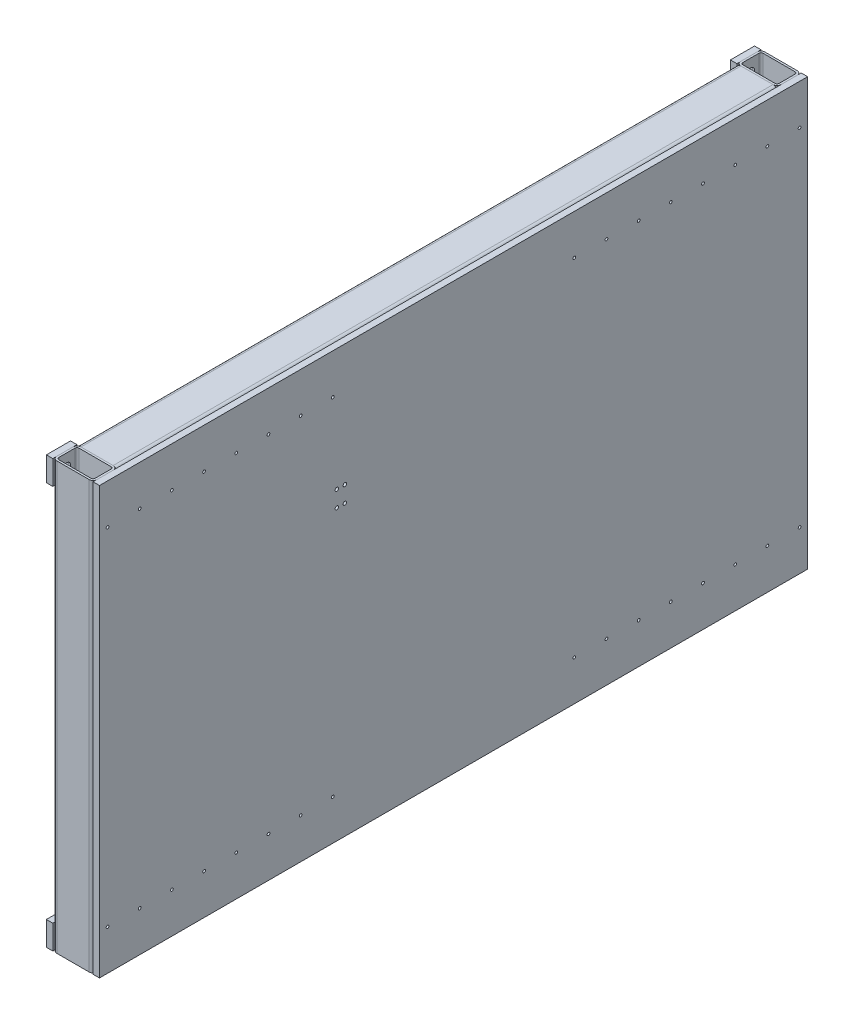
from build123d import *

# Parameters (mm, degrees)
F_100_X_60_X_5_0_1_DEPTH      = 1030
F_100_X_60_X_5_0_1_DEPTH_BACK = 30
F_100_X_60_X_5_0_1_2_DEPTH    = 1060
F_100_X_60_X_5_0_1_3_DEPTH    = 1702
F_100_X_60_X_5_0_1_4_DEPTH    = 1702
F_100_X_60_X_5_0_1_5_DEPTH    = 1702
F_100_X_60_X_5_0_1_6_DEPTH    = 1702
SKETCH_4_W                    = 1760
SKETCH_4_H                    = 1060
EXTRUDE_1_DEPTH               = 16
SKETCH_5_W                    = 60
SKETCH_5_H                    = 60
EXTRUDE_2_DEPTH               = 16
EXTRUDE_2_2_DEPTH             = 16
PATTERN_LINEAR_1_COUNT        = 8
PATTERN_LINEAR_1_PITCH        = 80
HOLE_WIZARD_M10_1_AT_2_COUNT  = 2
HOLE_WIZARD_M10_1_AT_2_PITCH  = 40
HOLE_WIZARD_M10_1_AT_3_COUNT  = 2
HOLE_WIZARD_M10_1_AT_3_PITCH  = 20
HOLE_WIZARD_M10_1_AT_4_COUNT  = 2
HOLE_WIZARD_M10_1_AT_4_PITCH  = 44.72135955


with BuildPart() as part:
    # Sketch1 → 矩型管 100 X 60 X 5.0(1) (new, two sides: drawn at the far end of the back side and taken through both)
    with BuildSketch(Plane(origin=(0, 500, 850), x_dir=(0, 0, -1), z_dir=(0, -1, 0)).offset(-F_100_X_60_X_5_0_1_DEPTH_BACK)):
        with BuildLine():
            Line((-20, -50), (20, -50))
            ThreePointArc((20, -50), (27.071067812, -47.071067812), (30, -40))
            Line((30, -40), (30, 40))
            ThreePointArc((30, 40), (27.071067812, 47.071067812), (20, 50))
            Line((20, 50), (-20, 50))
            ThreePointArc((-20, 50), (-27.071067812, 47.071067812), (-30, 40))
            Line((-30, 40), (-30, -40))
            ThreePointArc((-30, -40), (-27.071067812, -47.071067812), (-20, -50))
        make_face()
        with BuildLine():
            Line((-20, -45), (20, -45))
            ThreePointArc((20, -45), (23.535533906, -43.535533906), (25, -40))
            Line((25, -40), (25, 40))
            ThreePointArc((25, 40), (23.535533906, 43.535533906), (20, 45))
            Line((20, 45), (-20, 45))
            ThreePointArc((-20, 45), (-23.535533906, 43.535533906), (-25, 40))
            Line((-25, 40), (-25, -40))
            ThreePointArc((-25, -40), (-23.535533906, -43.535533906), (-20, -45))
        make_face(mode=Mode.SUBTRACT)
    extrude(amount=F_100_X_60_X_5_0_1_DEPTH + F_100_X_60_X_5_0_1_DEPTH_BACK)


with BuildPart() as body_2:
    # Sketch1 on segment 2 (carried to segment 2) → 100 X 60 X 5.0_1 2 (new body)
    with BuildSketch(Plane(origin=(0, 530, -850), x_dir=(0, 0, -1), z_dir=(0, -1, 0))):
        with BuildLine():
            Line((-20, -50), (20, -50))
            ThreePointArc((20, -50), (27.071067812, -47.071067812), (30, -40))
            Line((30, -40), (30, 40))
            ThreePointArc((30, 40), (27.071067812, 47.071067812), (20, 50))
            Line((20, 50), (-20, 50))
            ThreePointArc((-20, 50), (-27.071067812, 47.071067812), (-30, 40))
            Line((-30, 40), (-30, -40))
            ThreePointArc((-30, -40), (-27.071067812, -47.071067812), (-20, -50))
        make_face()
        with BuildLine():
            Line((-20, -45), (20, -45))
            ThreePointArc((20, -45), (23.535533906, -43.535533906), (25, -40))
            Line((25, -40), (25, 40))
            ThreePointArc((25, 40), (23.535533906, 43.535533906), (20, 45))
            Line((20, 45), (-20, 45))
            ThreePointArc((-20, 45), (-23.535533906, 43.535533906), (-25, 40))
            Line((-25, 40), (-25, -40))
            ThreePointArc((-25, -40), (-23.535533906, -43.535533906), (-20, -45))
        make_face(mode=Mode.SUBTRACT)
    extrude(amount=F_100_X_60_X_5_0_1_2_DEPTH)


with BuildPart() as body_3:
    # Sketch1 on segment 3 (carried to segment 3) → 100 X 60 X 5.0_1 3 (new body)
    with BuildSketch(Plane(origin=(0, -500, 851), x_dir=(0, 1, 0), z_dir=(0, 0, -1))):
        with BuildLine():
            Line((-20, -50), (20, -50))
            ThreePointArc((20, -50), (27.071067812, -47.071067812), (30, -40))
            Line((30, -40), (30, 40))
            ThreePointArc((30, 40), (27.071067812, 47.071067812), (20, 50))
            Line((20, 50), (-20, 50))
            ThreePointArc((-20, 50), (-27.071067812, 47.071067812), (-30, 40))
            Line((-30, 40), (-30, -40))
            ThreePointArc((-30, -40), (-27.071067812, -47.071067812), (-20, -50))
        make_face()
        with BuildLine():
            Line((-20, -45), (20, -45))
            ThreePointArc((20, -45), (23.535533906, -43.535533906), (25, -40))
            Line((25, -40), (25, 40))
            ThreePointArc((25, 40), (23.535533906, 43.535533906), (20, 45))
            Line((20, 45), (-20, 45))
            ThreePointArc((-20, 45), (-23.535533906, 43.535533906), (-25, 40))
            Line((-25, 40), (-25, -40))
            ThreePointArc((-25, -40), (-23.535533906, -43.535533906), (-20, -45))
        make_face(mode=Mode.SUBTRACT)
    extrude(amount=F_100_X_60_X_5_0_1_3_DEPTH)

    # 100 X 60 X 5.0_1 3 end butt 1
    split(bisect_by=Plane(origin=(0, -500, 820), x_dir=(0, 1, 0), z_dir=(0, 0, -1)), keep=Keep.TOP)

    # 100 X 60 X 5.0_1 3 end butt 2
    split(bisect_by=Plane(origin=(0, -500, -820), x_dir=(0, -1, 0), z_dir=(0, 0, 1)), keep=Keep.TOP)


with BuildPart() as body_4:
    # Sketch1 on segment 4 (carried to segment 4) → 100 X 60 X 5.0_1 4 (new body)
    with BuildSketch(Plane(origin=(0, -200, 851), x_dir=(0, 1, 0), z_dir=(0, 0, -1))):
        with BuildLine():
            Line((-20, -50), (20, -50))
            ThreePointArc((20, -50), (27.071067812, -47.071067812), (30, -40))
            Line((30, -40), (30, 40))
            ThreePointArc((30, 40), (27.071067812, 47.071067812), (20, 50))
            Line((20, 50), (-20, 50))
            ThreePointArc((-20, 50), (-27.071067812, 47.071067812), (-30, 40))
            Line((-30, 40), (-30, -40))
            ThreePointArc((-30, -40), (-27.071067812, -47.071067812), (-20, -50))
        make_face()
        with BuildLine():
            Line((-20, -45), (20, -45))
            ThreePointArc((20, -45), (23.535533906, -43.535533906), (25, -40))
            Line((25, -40), (25, 40))
            ThreePointArc((25, 40), (23.535533906, 43.535533906), (20, 45))
            Line((20, 45), (-20, 45))
            ThreePointArc((-20, 45), (-23.535533906, 43.535533906), (-25, 40))
            Line((-25, 40), (-25, -40))
            ThreePointArc((-25, -40), (-23.535533906, -43.535533906), (-20, -45))
        make_face(mode=Mode.SUBTRACT)
    extrude(amount=F_100_X_60_X_5_0_1_4_DEPTH)

    # 100 X 60 X 5.0_1 4 end butt 1
    split(bisect_by=Plane(origin=(0, -200, 820), x_dir=(0, 1, 0), z_dir=(0, 0, -1)), keep=Keep.TOP)

    # 100 X 60 X 5.0_1 4 end butt 2
    split(bisect_by=Plane(origin=(0, -200, -820), x_dir=(0, -1, 0), z_dir=(0, 0, 1)), keep=Keep.TOP)


with BuildPart() as body_5:
    # Sketch1 on segment 5 (carried to segment 5) → 100 X 60 X 5.0_1 5 (new body)
    with BuildSketch(Plane(origin=(0, 200, 851), x_dir=(0, 1, 0), z_dir=(0, 0, -1))):
        with BuildLine():
            Line((-20, -50), (20, -50))
            ThreePointArc((20, -50), (27.071067812, -47.071067812), (30, -40))
            Line((30, -40), (30, 40))
            ThreePointArc((30, 40), (27.071067812, 47.071067812), (20, 50))
            Line((20, 50), (-20, 50))
            ThreePointArc((-20, 50), (-27.071067812, 47.071067812), (-30, 40))
            Line((-30, 40), (-30, -40))
            ThreePointArc((-30, -40), (-27.071067812, -47.071067812), (-20, -50))
        make_face()
        with BuildLine():
            Line((-20, -45), (20, -45))
            ThreePointArc((20, -45), (23.535533906, -43.535533906), (25, -40))
            Line((25, -40), (25, 40))
            ThreePointArc((25, 40), (23.535533906, 43.535533906), (20, 45))
            Line((20, 45), (-20, 45))
            ThreePointArc((-20, 45), (-23.535533906, 43.535533906), (-25, 40))
            Line((-25, 40), (-25, -40))
            ThreePointArc((-25, -40), (-23.535533906, -43.535533906), (-20, -45))
        make_face(mode=Mode.SUBTRACT)
    extrude(amount=F_100_X_60_X_5_0_1_5_DEPTH)

    # 100 X 60 X 5.0_1 5 end butt 1
    split(bisect_by=Plane(origin=(0, 200, 820), x_dir=(0, 1, 0), z_dir=(0, 0, -1)), keep=Keep.TOP)

    # 100 X 60 X 5.0_1 5 end butt 2
    split(bisect_by=Plane(origin=(0, 200, -820), x_dir=(0, -1, 0), z_dir=(0, 0, 1)), keep=Keep.TOP)


with BuildPart() as body_6:
    # Sketch1 on segment 6 (carried to segment 6) → 100 X 60 X 5.0_1 6 (new body)
    with BuildSketch(Plane(origin=(0, 500, 851), x_dir=(0, 1, 0), z_dir=(0, 0, -1))):
        with BuildLine():
            Line((-20, -50), (20, -50))
            ThreePointArc((20, -50), (27.071067812, -47.071067812), (30, -40))
            Line((30, -40), (30, 40))
            ThreePointArc((30, 40), (27.071067812, 47.071067812), (20, 50))
            Line((20, 50), (-20, 50))
            ThreePointArc((-20, 50), (-27.071067812, 47.071067812), (-30, 40))
            Line((-30, 40), (-30, -40))
            ThreePointArc((-30, -40), (-27.071067812, -47.071067812), (-20, -50))
        make_face()
        with BuildLine():
            Line((-20, -45), (20, -45))
            ThreePointArc((20, -45), (23.535533906, -43.535533906), (25, -40))
            Line((25, -40), (25, 40))
            ThreePointArc((25, 40), (23.535533906, 43.535533906), (20, 45))
            Line((20, 45), (-20, 45))
            ThreePointArc((-20, 45), (-23.535533906, 43.535533906), (-25, 40))
            Line((-25, 40), (-25, -40))
            ThreePointArc((-25, -40), (-23.535533906, -43.535533906), (-20, -45))
        make_face(mode=Mode.SUBTRACT)
    extrude(amount=F_100_X_60_X_5_0_1_6_DEPTH)

    # 100 X 60 X 5.0_1 6 end butt 1
    split(bisect_by=Plane(origin=(0, 500, 820), x_dir=(0, 1, 0), z_dir=(0, 0, -1)), keep=Keep.TOP)

    # 100 X 60 X 5.0_1 6 end butt 2
    split(bisect_by=Plane(origin=(0, 500, -820), x_dir=(0, -1, 0), z_dir=(0, 0, 1)), keep=Keep.TOP)


with BuildPart() as body_7:
    # 草图4 → 凸台-拉伸1 (new body)
    with BuildSketch(Plane(origin=(50, 0, 0), x_dir=(0, 0, -1), z_dir=(1, 0, 0))):
        Rectangle(SKETCH_4_W, SKETCH_4_H)
    extrude(amount=EXTRUDE_1_DEPTH)


with BuildPart() as body_8:
    # 草图5 → 凸台-拉伸2 (new body)
    with BuildSketch(Plane.ZY.offset(50)):
        with Locations((-850, 500)):
            Rectangle(SKETCH_5_W, SKETCH_5_H)
    extrude_2 = extrude(amount=EXTRUDE_2_DEPTH)


with BuildPart() as body_9:
    # 草图5 → Extrude 2 2 (new body)
    with BuildSketch(Plane.ZY.offset(50)):
        with Locations((850, 500)):
            Rectangle(SKETCH_5_W, SKETCH_5_H)
    extrude_2_2 = extrude(amount=EXTRUDE_2_2_DEPTH)


with BuildPart() as part_1:
    add(part.part)

    add(body_2.part)  # 镜向3 merges body 2
    # 镜向3: 凸台-拉伸2, Extrude 2 2 across plane
    add(extrude_2.mirror(Plane.ZX))
    add(extrude_2_2.mirror(Plane.ZX))

    # 草图8 → M20 螺纹孔1 (revolve, cut)
    with BuildSketch(Plane(origin=(-66, -500, -850), x_dir=(0, 0, 1), z_dir=(0, 1, 0))):
        Polygon((0, 0), (0, 52.757530416), (8.75, 47.5), (8.75, 0), align=None)
    hole_wizard_m20_1 = revolve(axis=Axis((-72.35, -500, -850), (1, 0, 0)), mode=Mode.SUBTRACT)


with BuildPart() as mirror_9_tool:
    # 镜向9: M20 螺纹孔1 across plane
    add(hole_wizard_m20_1.mirror(Plane.ZX))


with BuildPart() as part_2:
    add(part_1.part)

    # 镜向9: cut by mirror_9_tool
    add(mirror_9_tool.part, mode=Mode.SUBTRACT)

    # 镜向11: M20 螺纹孔1 across plane
    add(hole_wizard_m20_1.mirror(Plane.XY), mode=Mode.SUBTRACT)


with BuildPart() as body_8_1:
    add(body_8.part)

    # 镜向9: cut by mirror_9_tool
    add(mirror_9_tool.part, mode=Mode.SUBTRACT)


with BuildPart() as mirror_11_copy_1_tool:
    # 镜向11 copy 1 sketch → 镜向11 copy 1 (revolve)
    with BuildSketch(Plane(origin=(-66, 500, 850), x_dir=(0, 0, -1), z_dir=(0, -1, 0))):
        Polygon((0, 0), (0, 52.757530416), (8.75, 47.5), (8.75, 0), align=None)
    revolve(axis=Axis((-72.35, 500, 850), (1, 0, 0)))


with BuildPart() as part_3:
    add(part_2.part)

    # 镜向11 copy 1: cut by mirror_11_copy_1_tool
    add(mirror_11_copy_1_tool.part, mode=Mode.SUBTRACT)


with BuildPart() as body_9_1:
    add(body_9.part)

    # 镜向11 copy 1: cut by mirror_11_copy_1_tool
    add(mirror_11_copy_1_tool.part, mode=Mode.SUBTRACT)


with BuildPart() as hole_wizard_m8_1_tool:
    # 草图10 → M8 螺纹孔1 (revolve)
    with BuildSketch(Plane(origin=(66, 430, 860), x_dir=(0, 0, -1), z_dir=(0, 1, 0))):
        Polygon((0, 0), (0, 21.792926105), (3.4, 19.75), (3.4, 0), align=None)
    hole_wizard_m8_1 = revolve(axis=Axis((72.35, 430, 860), (-1, 0, 0)))


with BuildPart() as part_4:
    add(part_3.part)

    # M8 螺纹孔1: cut by hole_wizard_m8_1_tool
    add(hole_wizard_m8_1_tool.part, mode=Mode.SUBTRACT)


with BuildPart() as body_7_1:
    add(body_7.part)

    # M8 螺纹孔1: cut by hole_wizard_m8_1_tool
    add(hole_wizard_m8_1_tool.part, mode=Mode.SUBTRACT)

    # 阵列(线性)1: M8 螺纹孔1 ×8
    with Locations(*[(0, 0, -i * PATTERN_LINEAR_1_PITCH) for i in range(1, PATTERN_LINEAR_1_COUNT)]):
        add(hole_wizard_m8_1, mode=Mode.SUBTRACT)

    # 镜向12: M8 螺纹孔1 across plane
    add(hole_wizard_m8_1.mirror(Plane.ZX), mode=Mode.SUBTRACT)

    # 镜向12 copy 1 sketch → 镜向12 copy 1 (revolve, cut)
    with BuildSketch(Plane(origin=(66, -430, 780), x_dir=(0, 0, -1), z_dir=(0, -1, 0))):
        Polygon((0, 0), (0, -21.792926105), (3.4, -19.75), (3.4, 0), align=None)
    revolve(axis=Axis((72.35, -430, 780), (1, 0, 0)), mode=Mode.SUBTRACT)

    # 镜向12 copy 2 sketch → 镜向12 copy 2 (revolve, cut)
    with BuildSketch(Plane(origin=(66, -430, 700), x_dir=(0, 0, -1), z_dir=(0, -1, 0))):
        Polygon((0, 0), (0, -21.792926105), (3.4, -19.75), (3.4, 0), align=None)
    revolve(axis=Axis((72.35, -430, 700), (1, 0, 0)), mode=Mode.SUBTRACT)

    # 镜向12 copy 3 sketch → 镜向12 copy 3 (revolve, cut)
    with BuildSketch(Plane(origin=(66, -430, 620), x_dir=(0, 0, -1), z_dir=(0, -1, 0))):
        Polygon((0, 0), (0, -21.792926105), (3.4, -19.75), (3.4, 0), align=None)
    revolve(axis=Axis((72.35, -430, 620), (1, 0, 0)), mode=Mode.SUBTRACT)

    # 镜向12 copy 4 sketch → 镜向12 copy 4 (revolve, cut)
    with BuildSketch(Plane(origin=(66, -430, 540), x_dir=(0, 0, -1), z_dir=(0, -1, 0))):
        Polygon((0, 0), (0, -21.792926105), (3.4, -19.75), (3.4, 0), align=None)
    revolve(axis=Axis((72.35, -430, 540), (1, 0, 0)), mode=Mode.SUBTRACT)

    # 镜向12 copy 5 sketch → 镜向12 copy 5 (revolve, cut)
    with BuildSketch(Plane(origin=(66, -430, 460), x_dir=(0, 0, -1), z_dir=(0, -1, 0))):
        Polygon((0, 0), (0, -21.792926105), (3.4, -19.75), (3.4, 0), align=None)
    revolve(axis=Axis((72.35, -430, 460), (1, 0, 0)), mode=Mode.SUBTRACT)

    # 镜向12 copy 6 sketch → 镜向12 copy 6 (revolve, cut)
    with BuildSketch(Plane(origin=(66, -430, 380), x_dir=(0, 0, -1), z_dir=(0, -1, 0))):
        Polygon((0, 0), (0, -21.792926105), (3.4, -19.75), (3.4, 0), align=None)
    revolve(axis=Axis((72.35, -430, 380), (1, 0, 0)), mode=Mode.SUBTRACT)

    # 镜向12 copy 7 sketch → 镜向12 copy 7 (revolve, cut)
    with BuildSketch(Plane(origin=(66, -430, 300), x_dir=(0, 0, -1), z_dir=(0, -1, 0))):
        Polygon((0, 0), (0, -21.792926105), (3.4, -19.75), (3.4, 0), align=None)
    revolve(axis=Axis((72.35, -430, 300), (1, 0, 0)), mode=Mode.SUBTRACT)

    # 镜向13: M8 螺纹孔1 across plane
    add(hole_wizard_m8_1.mirror(Plane.XY), mode=Mode.SUBTRACT)

    # 镜向13 copy 1 sketch → 镜向13 copy 1 (revolve, cut)
    with BuildSketch(Plane(origin=(66, 430, -780), x_dir=(0, 0, 1), z_dir=(0, 1, 0))):
        Polygon((0, 0), (0, -21.792926105), (3.4, -19.75), (3.4, 0), align=None)
    revolve(axis=Axis((72.35, 430, -780), (1, 0, 0)), mode=Mode.SUBTRACT)

    # 镜向13 copy 2 sketch → 镜向13 copy 2 (revolve, cut)
    with BuildSketch(Plane(origin=(66, 430, -700), x_dir=(0, 0, 1), z_dir=(0, 1, 0))):
        Polygon((0, 0), (0, -21.792926105), (3.4, -19.75), (3.4, 0), align=None)
    revolve(axis=Axis((72.35, 430, -700), (1, 0, 0)), mode=Mode.SUBTRACT)

    # 镜向13 copy 3 sketch → 镜向13 copy 3 (revolve, cut)
    with BuildSketch(Plane(origin=(66, 430, -620), x_dir=(0, 0, 1), z_dir=(0, 1, 0))):
        Polygon((0, 0), (0, -21.792926105), (3.4, -19.75), (3.4, 0), align=None)
    revolve(axis=Axis((72.35, 430, -620), (1, 0, 0)), mode=Mode.SUBTRACT)

    # 镜向13 copy 4 sketch → 镜向13 copy 4 (revolve, cut)
    with BuildSketch(Plane(origin=(66, 430, -540), x_dir=(0, 0, 1), z_dir=(0, 1, 0))):
        Polygon((0, 0), (0, -21.792926105), (3.4, -19.75), (3.4, 0), align=None)
    revolve(axis=Axis((72.35, 430, -540), (1, 0, 0)), mode=Mode.SUBTRACT)

    # 镜向13 copy 5 sketch → 镜向13 copy 5 (revolve, cut)
    with BuildSketch(Plane(origin=(66, 430, -460), x_dir=(0, 0, 1), z_dir=(0, 1, 0))):
        Polygon((0, 0), (0, -21.792926105), (3.4, -19.75), (3.4, 0), align=None)
    revolve(axis=Axis((72.35, 430, -460), (1, 0, 0)), mode=Mode.SUBTRACT)

    # 镜向13 copy 6 sketch → 镜向13 copy 6 (revolve, cut)
    with BuildSketch(Plane(origin=(66, 430, -380), x_dir=(0, 0, 1), z_dir=(0, 1, 0))):
        Polygon((0, 0), (0, -21.792926105), (3.4, -19.75), (3.4, 0), align=None)
    revolve(axis=Axis((72.35, 430, -380), (1, 0, 0)), mode=Mode.SUBTRACT)

    # 镜向13 copy 7 sketch → 镜向13 copy 7 (revolve, cut)
    with BuildSketch(Plane(origin=(66, 430, -300), x_dir=(0, 0, 1), z_dir=(0, 1, 0))):
        Polygon((0, 0), (0, -21.792926105), (3.4, -19.75), (3.4, 0), align=None)
    revolve(axis=Axis((72.35, 430, -300), (1, 0, 0)), mode=Mode.SUBTRACT)

    # 镜向13 copy 8 sketch → 镜向13 copy 8 (revolve, cut)
    with BuildSketch(Plane(origin=(66, -430, -860), x_dir=(0, 0, 1), z_dir=(0, -1, 0))):
        Polygon((0, 0), (0, 21.792926105), (3.4, 19.75), (3.4, 0), align=None)
    revolve(axis=Axis((72.35, -430, -860), (-1, 0, 0)), mode=Mode.SUBTRACT)

    # 镜向13 copy 9 sketch → 镜向13 copy 9 (revolve, cut)
    with BuildSketch(Plane(origin=(66, -430, -780), x_dir=(0, 0, 1), z_dir=(0, -1, 0))):
        Polygon((0, 0), (0, 21.792926105), (3.4, 19.75), (3.4, 0), align=None)
    revolve(axis=Axis((72.35, -430, -780), (-1, 0, 0)), mode=Mode.SUBTRACT)

    # 镜向13 copy 10 sketch → 镜向13 copy 10 (revolve, cut)
    with BuildSketch(Plane(origin=(66, -430, -700), x_dir=(0, 0, 1), z_dir=(0, -1, 0))):
        Polygon((0, 0), (0, 21.792926105), (3.4, 19.75), (3.4, 0), align=None)
    revolve(axis=Axis((72.35, -430, -700), (-1, 0, 0)), mode=Mode.SUBTRACT)

    # 镜向13 copy 11 sketch → 镜向13 copy 11 (revolve, cut)
    with BuildSketch(Plane(origin=(66, -430, -620), x_dir=(0, 0, 1), z_dir=(0, -1, 0))):
        Polygon((0, 0), (0, 21.792926105), (3.4, 19.75), (3.4, 0), align=None)
    revolve(axis=Axis((72.35, -430, -620), (-1, 0, 0)), mode=Mode.SUBTRACT)

    # 镜向13 copy 12 sketch → 镜向13 copy 12 (revolve, cut)
    with BuildSketch(Plane(origin=(66, -430, -540), x_dir=(0, 0, 1), z_dir=(0, -1, 0))):
        Polygon((0, 0), (0, 21.792926105), (3.4, 19.75), (3.4, 0), align=None)
    revolve(axis=Axis((72.35, -430, -540), (-1, 0, 0)), mode=Mode.SUBTRACT)

    # 镜向13 copy 13 sketch → 镜向13 copy 13 (revolve, cut)
    with BuildSketch(Plane(origin=(66, -430, -460), x_dir=(0, 0, 1), z_dir=(0, -1, 0))):
        Polygon((0, 0), (0, 21.792926105), (3.4, 19.75), (3.4, 0), align=None)
    revolve(axis=Axis((72.35, -430, -460), (-1, 0, 0)), mode=Mode.SUBTRACT)

    # 镜向13 copy 14 sketch → 镜向13 copy 14 (revolve, cut)
    with BuildSketch(Plane(origin=(66, -430, -380), x_dir=(0, 0, 1), z_dir=(0, -1, 0))):
        Polygon((0, 0), (0, 21.792926105), (3.4, 19.75), (3.4, 0), align=None)
    revolve(axis=Axis((72.35, -430, -380), (-1, 0, 0)), mode=Mode.SUBTRACT)

    # 镜向13 copy 15 sketch → 镜向13 copy 15 (revolve, cut)
    with BuildSketch(Plane(origin=(66, -430, -300), x_dir=(0, 0, 1), z_dir=(0, -1, 0))):
        Polygon((0, 0), (0, 21.792926105), (3.4, 19.75), (3.4, 0), align=None)
    revolve(axis=Axis((72.35, -430, -300), (-1, 0, 0)), mode=Mode.SUBTRACT)

    # 草图12 → M10 螺纹孔1 (revolve, cut)
    with BuildSketch(Plane(origin=(66, 227, 270.25), x_dir=(0, 0, -1), z_dir=(0, 1, 0))):
        Polygon((0, 0), (0, 42.553657631), (4.25, 40), (4.25, 0), align=None)
    hole_wizard_m10_1 = revolve(axis=Axis((72.35, 227, 270.25), (-1, 0, 0)), mode=Mode.SUBTRACT)

    # M10 螺纹孔1 at 2: M10 螺纹孔1 ×2
    with Locations(*[(0, -i * HOLE_WIZARD_M10_1_AT_2_PITCH, 0) for i in range(1, HOLE_WIZARD_M10_1_AT_2_COUNT)]):
        add(hole_wizard_m10_1, mode=Mode.SUBTRACT)

    # M10 螺纹孔1 at 3: M10 螺纹孔1 ×2
    with Locations(*[(0, 0, i * HOLE_WIZARD_M10_1_AT_3_PITCH) for i in range(1, HOLE_WIZARD_M10_1_AT_3_COUNT)]):
        add(hole_wizard_m10_1, mode=Mode.SUBTRACT)

    # M10 螺纹孔1 at 4: M10 螺纹孔1 ×2
    with Locations(*[Vector(0, -0.894427190999916, 0.447213595499958) * (i * HOLE_WIZARD_M10_1_AT_4_PITCH) for i in range(1, HOLE_WIZARD_M10_1_AT_4_COUNT)]):
        add(hole_wizard_m10_1, mode=Mode.SUBTRACT)


solid = Compound([body_3.part, body_4.part, body_5.part, body_6.part, body_8_1.part, body_9_1.part, part_4.part, body_7_1.part])
